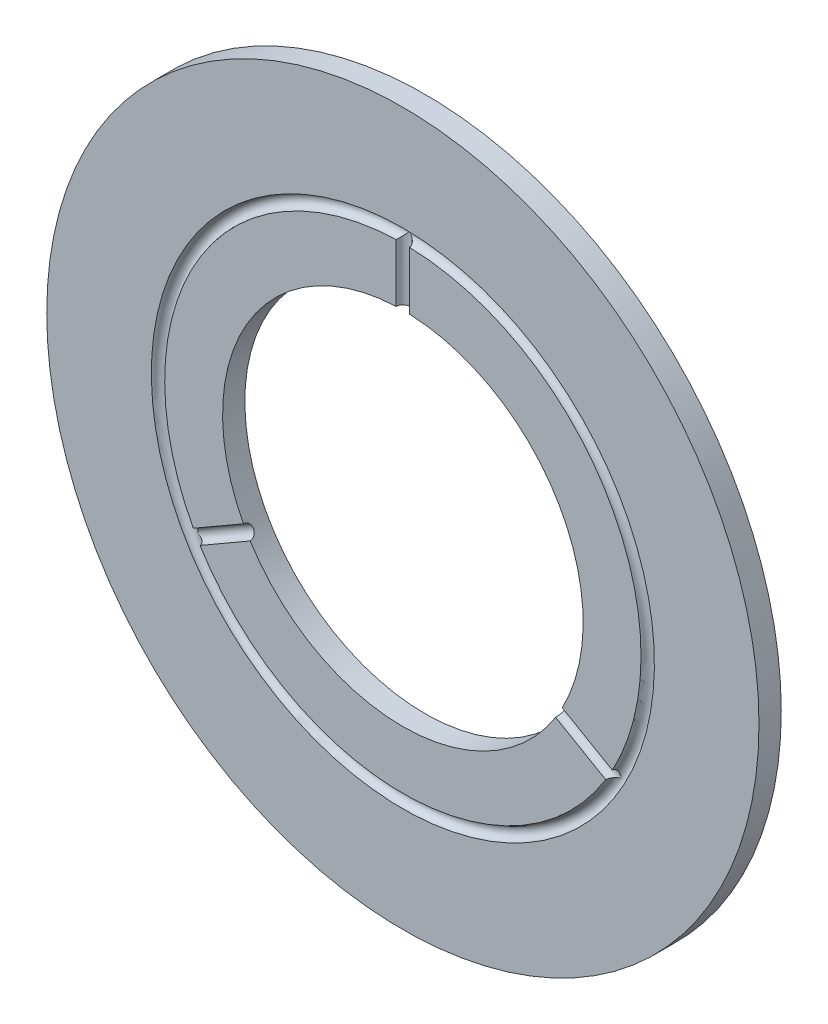
SolidWorks part; units mm, degrees
material "黄铜"
ref_plane "前视基准面" through (0, 0, 0) normal (0, 0, 1) x (1, 0, 0)
ref_plane "上视基准面" through (0, 0, 0) normal (0, 1, 0) x (1, 0, 0)
ref_plane "右视基准面" through (0, 0, 0) normal (1, 0, 0) x (0, 0, -1)
sketch "草图1" plane through (0, 0, 0) normal (0, 0, 1) x (1, 0, 0)
  circle A0 centre (0, 0) radius 40.5
  circle A1 centre (0, 0) radius 80
  dimension "D1" = 81
  dimension "D2" = 160
extrude "凸台-拉伸1" add sketch "草图1" along normal blind 5
sketch "草图2" plane through (0, 0, 5) normal (0, 0, 1) x (1, 0, 0)
  circle A0 centre (0, 0) radius 55
  dimension "D1" = 110
sketch "草图3" plane through (0, 0, 0) normal (1, 0, 0) x (0, 0, -1)
  line L0 (-5, 55) -> (-5, -55) construction
  line L1 (-5, 80) -> (-5, -80) construction
  line L2 (-5, 55) -> (-5, 0) construction
  circle A0 centre (-5, 55) radius 1.5
  dimension "D1" = 3
  dimension "D2" = 55
sweep "切除-扫描1" cut profiles "草图3" path "草图2"
sketch "草图5" plane through (0, 0, 0) normal (0, 1, 0) x (1, 0, 0)
  line L0 (-80, -5) -> (80, -5) construction
  circle A0 centre (0, -5) radius 1.5
  dimension "D1" = 3
extrude "切除-拉伸2" cut sketch "草图5" along normal blind 55
pattern_circular "阵列(圆周)1" count 3 over 360 about axis through (0, 0, 5) along (0, 0, -1) of "切除-拉伸2"
